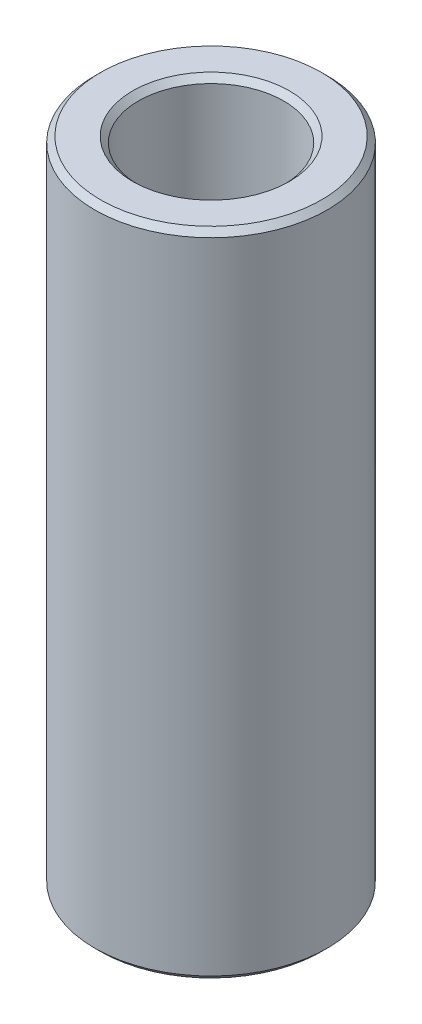
SolidWorks part; units mm, degrees
material "Brass"
ref_plane "Front Plane" through (0, 0, 0) normal (0, 0, 1) x (1, 0, 0)
ref_plane "Top Plane" through (0, 0, 0) normal (0, 1, 0) x (1, 0, 0)
ref_plane "Right Plane" through (0, 0, 0) normal (1, 0, 0) x (0, 0, -1)
sketch "Sketch1" plane through (0, 0, 0) normal (0, 1, 0) x (1, 0, 0)
  circle A0 centre (0, 0) radius 12.5
  circle A1 centre (0, 0) radius 20
  dimension "D1" = 25
  dimension "D2" = 40
extrude "Boss-Extrude1" add sketch "Sketch1" along normal blind 112
chamfer "Chamfer1" distance 1 angle 45 4 edges at (0, 0, 20) (0, 112, 20) (0, 0, 12.5) (0, 112, 12.5)
